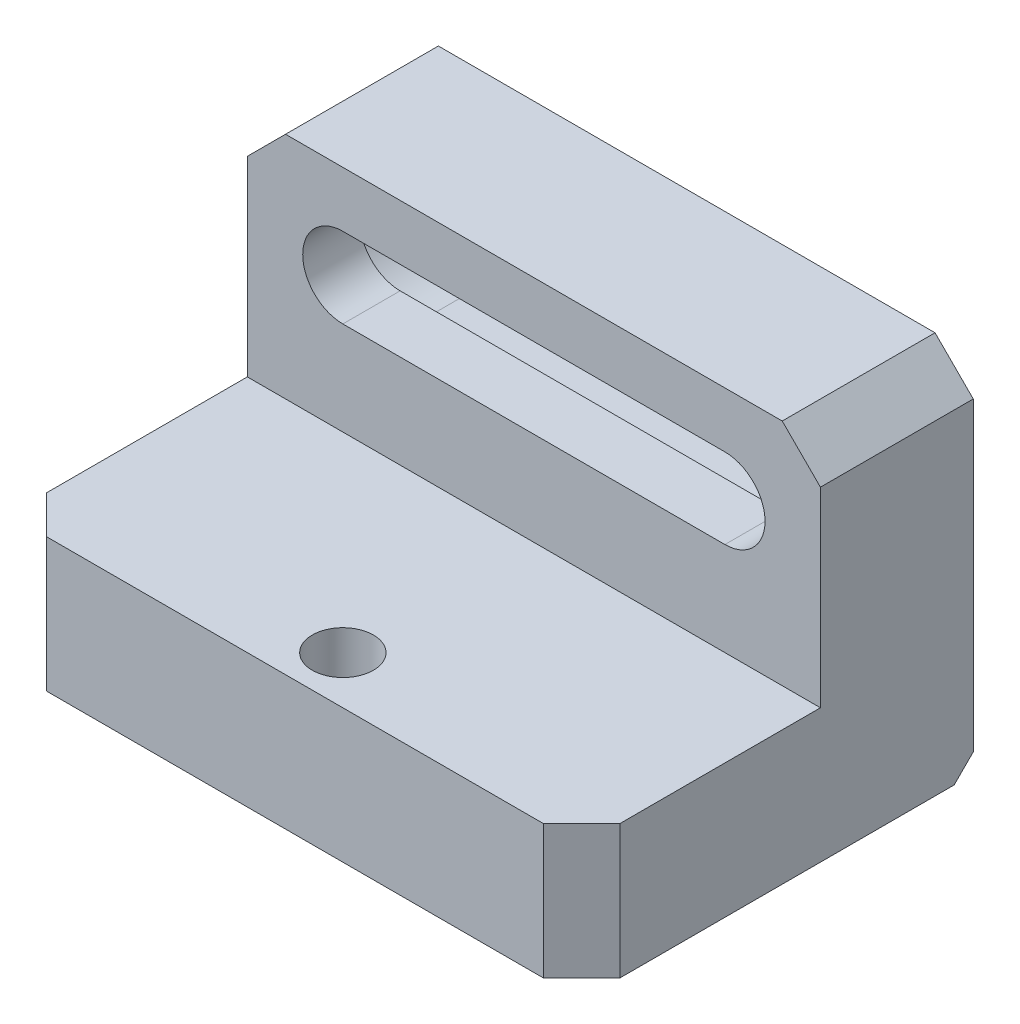
SolidWorks part; units mm, degrees
ref_plane "前视基准面" through (0, 0, 0) normal (0, 0, 1) x (1, 0, 0)
ref_plane "上视基准面" through (0, 0, 0) normal (0, 1, 0) x (1, 0, 0)
ref_plane "右视基准面" through (0, 0, 0) normal (1, 0, 0) x (0, 0, -1)
sketch "草图1" plane through (0, 0, 0) normal (0, 0, 1) x (1, 0, 0)
  line L1 (-15, -9.5) -> (15, -9.5)
  line L2 (-15, -9.5) -> (-15, 9.5)
  line L3 (-15, 9.5) -> (15, 9.5)
  line L4 (15, -9.5) -> (15, 9.5)
  line L5 (-15, -9.5) -> (15, 9.5) construction
  line L6 (-15, 9.5) -> (15, -9.5) construction
  point P0 (0, 0)
  dimension "D1" = 19
  dimension "D2" = 30
extrude "凸台-拉伸1" add sketch "草图1" along normal blind 20.5
sketch "草图2" plane through (0, 0, 20.5) normal (0, 0, 1) x (1, 0, 0)
  line L0 (15, -9.5) -> (15, 9.5) construction
  line L1 (-15, 9.5) -> (15, 9.5)
  line L2 (-15, 9.5) -> (-15, -2.5)
  line L3 (-15, -2.5) -> (15, -2.5)
  line L4 (15, 9.5) -> (15, -2.5)
  dimension "D1" = 12
extrude "切除-拉伸1" cut sketch "草图2" against normal blind 12.5
sketch "草图3" plane through (0, 0, 0) normal (0, 0, -1) x (-1, 0, 0)
  line L0 (10, 4.5) -> (-10, 4.5) construction
  line L1 (10, 2.4) -> (-10, 2.4)
  line L2 (10, 6.6) -> (-10, 6.6)
  line L3 (0, 9.5) -> (0, 4.5) construction
  line L4 (-15, 9.5) -> (15, 9.5) construction
  arc A0 (10, 2.4) -> (10, 6.6) centre (10, 4.5) ccw
  arc A1 (-10, 6.6) -> (-10, 2.4) centre (-10, 4.5) ccw
  point P2 (0, 4.5)
  dimension "D1" = 5
  dimension "D2" = 20
  dimension "D3" = 4.2
extrude "切除-拉伸2" cut sketch "草图3" against normal through all
sketch "草图4" plane through (0, 0, 0) normal (0, 0, -1) x (-1, 0, 0)
  line L0 (10, 4.5) -> (-10, 4.5) construction
  line L1 (10, 0.5) -> (-10, 0.5)
  line L2 (10, 8.5) -> (-10, 8.5)
  arc A0 (10, 0.5) -> (10, 8.5) centre (10, 4.5) ccw
  arc A1 (-10, 8.5) -> (-10, 0.5) centre (-10, 4.5) ccw
  point P4 (0, 4.5)
  dimension "D1" = 8
extrude "切除-拉伸3" cut sketch "草图4" against normal blind 5
sketch "草图5" plane through (0, 0, 0) normal (0, 0, -1) x (-1, 0, 0)
  line L0 (0, 0) -> (0, -6) construction
  line L1 (15, -9.5) -> (-15, -9.5) construction
  circle A0 centre (0, -6) radius 1.75
  dimension "D1" = 3.5
  dimension "D2" = 3.5
extrude "切除-拉伸4" cut sketch "草图5" against normal blind 10
hole_wizard "M3 间隙孔1" positions "草图6" profile "草图7" hole size "M3" standard "GB" end condition through all
sketch "草图6" plane through (0, -9.5, 0) normal (0, -1, 0) x (-1, 0, 0)
  line L0 (0, -20.5) -> (0, -18) construction
  line L1 (15, -20.5) -> (-15, -20.5) construction
  point P0 (0, -18)
  dimension "D1" = 2.5
sketch "草图7" plane through (0, -9.5, 18) normal (1, 0, 0) x (0, 0, -1)
  line L0 (0, 0) -> (0, 19)
  line L1 (0, 19) -> (1.6, 19)
  line L2 (1.6, 19) -> (1.6, 0)
  line L5 (1.6, 0) -> (0, 0)
  line L11 (0, -6.35) -> (0, 107.95) construction
  dimension "通孔孔直径" = 3.2
  dimension "通孔孔深度" = 19
hole_wizard "M3 螺纹孔1" positions "草图8" profile "草图9" tap size "M3" standard "GB"
sketch "草图8" plane through (0, 0, 10) normal (0, 0, -1) x (-1, 0, 0)
  point P0 (0, -6)
sketch "草图9" plane through (0, -6, 10) normal (1, 0, 0) x (0, 1, 0)
  line L0 (0, 0) -> (0, 6.4)
  line L1 (0, 6.4) -> (1.25, 6.4)
  line L2 (1.25, 6.4) -> (1.25, 0)
  line L5 (1.25, 0) -> (0, 0)
  line L11 (0, -6.35) -> (0, 107.95) construction
  dimension "通孔螺纹孔钻头直径" = 2.5
  dimension "通孔螺纹孔钻头深度" = 6.4
cosmetic thread "孔螺蚊线1" parameters "D2"=3
chamfer "倒角1" distance 2 angle 45 4 edges at (-15, 9.5, 4) (15, 9.5, 4) (15, -6, 20.5) (-15, -6, 20.5)
chamfer "倒角2" distance 1 angle 45 1 edges at (0, -9.5, 0)
